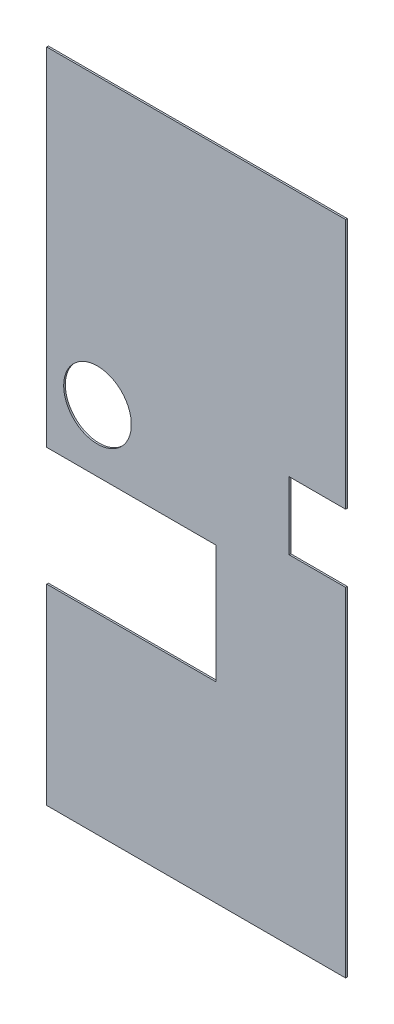
from build123d import *

# Parameters (mm, degrees)
BOSS_EXTRUDE1_DEPTH = 3
SKETCH2_R           = 60
SKETCH2_W           = 120
SKETCH2_H           = 120
CUT_EXTRUDE1_DEPTH  = 10


with BuildPart() as part:
    # Sketch1 → Boss-Extrude1 (new body)
    with BuildSketch(Plane.XY):
        Polygon((0, 0), (530, 0), (530, 1165), (0, 1165), (0, 550), (300, 550), (300, 340), (0, 340), align=None)
    extrude(amount=BOSS_EXTRUDE1_DEPTH)

    # Sketch2 → Cut-Extrude1 (cut)
    with BuildSketch(Plane(origin=(0, 0, 0), x_dir=(-1, 0, 0), z_dir=(0, 0, -1))):
        with Locations((-90, 660)):
            Circle(SKETCH2_R)
        with Locations((-490, 660)):
            Rectangle(SKETCH2_W, SKETCH2_H)
    extrude(amount=-CUT_EXTRUDE1_DEPTH, mode=Mode.SUBTRACT)


solid = part.part
